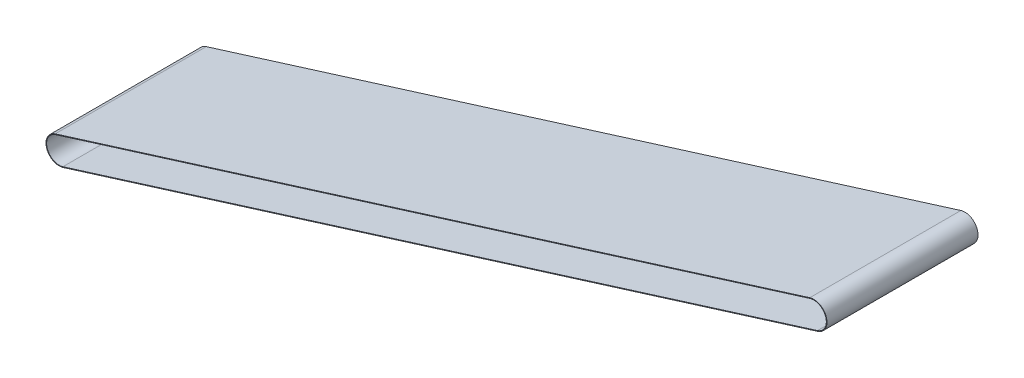
from build123d import *

# Parameters (mm, degrees)
EXTRUDE_1_DEPTH = 720


with BuildPart() as part:
    # 草图1 → 凸台-拉伸1 (new body)
    with BuildSketch(Plane.XY.offset(360)):
        with BuildLine():
            Line((-204.760757807, 647.741782203), (3391.739242193, 1769.641782203))
            ThreePointArc((3391.739242193, 1769.641782203), (3470.641782203, 1728.260757807), (3429.260757807, 1649.358217797))
            Line((3429.260757807, 1649.358217797), (-167.239242193, 527.458217797))
            ThreePointArc((-167.239242193, 527.458217797), (-246.141782203, 568.839242193), (-204.760757807, 647.741782203))
        make_face()
        with BuildLine():
            Line((-203.867388388, 644.877887812), (3392.632611612, 1766.777887812))
            ThreePointArc((3392.632611612, 1766.777887812), (3467.777887812, 1727.367388388), (3428.367388388, 1652.222112188))
            Line((3428.367388388, 1652.222112188), (-168.132611612, 530.322112188))
            ThreePointArc((-168.132611612, 530.322112188), (-243.277887812, 569.732611612), (-203.867388388, 644.877887812))
        make_face(mode=Mode.SUBTRACT)
    extrude(amount=-EXTRUDE_1_DEPTH)


solid = part.part
